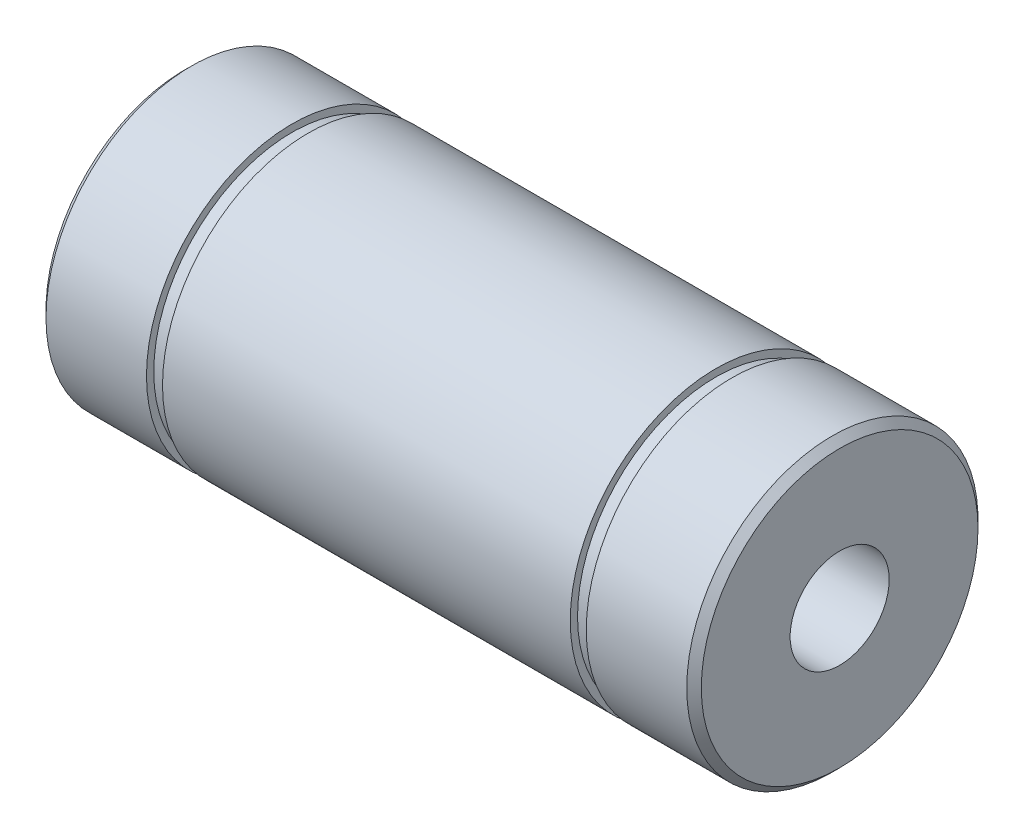
SolidWorks part; units mm, degrees
material "普通碳钢"
ref_plane "前视基准面" through (0, 0, 0) normal (0, 0, 1) x (1, 0, 0)
ref_plane "上视基准面" through (0, 0, 0) normal (0, 1, 0) x (1, 0, 0)
ref_plane "右视基准面" through (0, 0, 0) normal (1, 0, 0) x (0, 0, -1)
sketch "草图1" plane through (0, 0, 0) normal (1, 0, 0) x (0, 0, -1)
  circle A0 centre (0, 0) radius 10
  dimension "D1" = 20
extrude "凸台-拉伸1" add sketch "草图1" along normal mid plane 45
hole_wizard "M8 螺纹孔1" positions "草图3" profile "草图2" tap size "M8" standard "Gb"
sketch "草图3" plane through (22.5, 0, 0) normal (1, 0, 0) x (0, 0, -1)
  point P0 (0, 0)
sketch "草图2" plane through (22.5, 0, 0) normal (0, 1, 0) x (0, 0, -1)
  line L0 (0, 0) -> (0, 21.7929)
  line L1 (0, 21.7929) -> (3.4, 19.75)
  line L2 (3.4, 19.75) -> (3.4, 0)
  line L5 (3.4, 0) -> (0, 0)
  line L10 (0, 21.7929) -> (-3.4, 19.75) construction
  line L11 (0, -6.35) -> (0, 107.95) construction
  dimension "螺纹孔钻头直径" = 6.8
  dimension "螺纹孔钻头深度" = 19.75
  dimension "导头角度" = 118
cosmetic thread "孔螺蚊线1" parameters "D1"=16, "D2"=8
mirror "镜向1" about plane through (0, 0, 0) normal (1, 0, 0) of "M8 螺纹孔1"
chamfer "倒角1" distance 0.5 angle 45 2 edges at (22.5, 0, -10) (-22.5, 0, -10)
sketch "草图4" plane through (0, 0, 0) normal (0, 0, 1) x (1, 0, 0)
  line L0 (22, 10) -> (-22, 10) construction
  line L1 (-15.1, 10) -> (-14, 10)
  line L2 (-15.1, 10) -> (-15.1, 9.5)
  line L3 (-15.1, 9.5) -> (-14, 9.5)
  line L4 (-14, 10) -> (-14, 9.5)
  line L5 (0, 13.4045) -> (0, 0) construction
  line L6 (0, 0) -> (28.5756, 0) construction
  dimension "D1" = 14
  dimension "D2" = 1.1
  dimension "D3" = 9.5
revolve "切除-旋转1" cut sketch "草图4" angle 360 about L6
mirror "镜向2" about plane through (0, 0, 0) normal (1, 0, 0) of "切除-旋转1"
